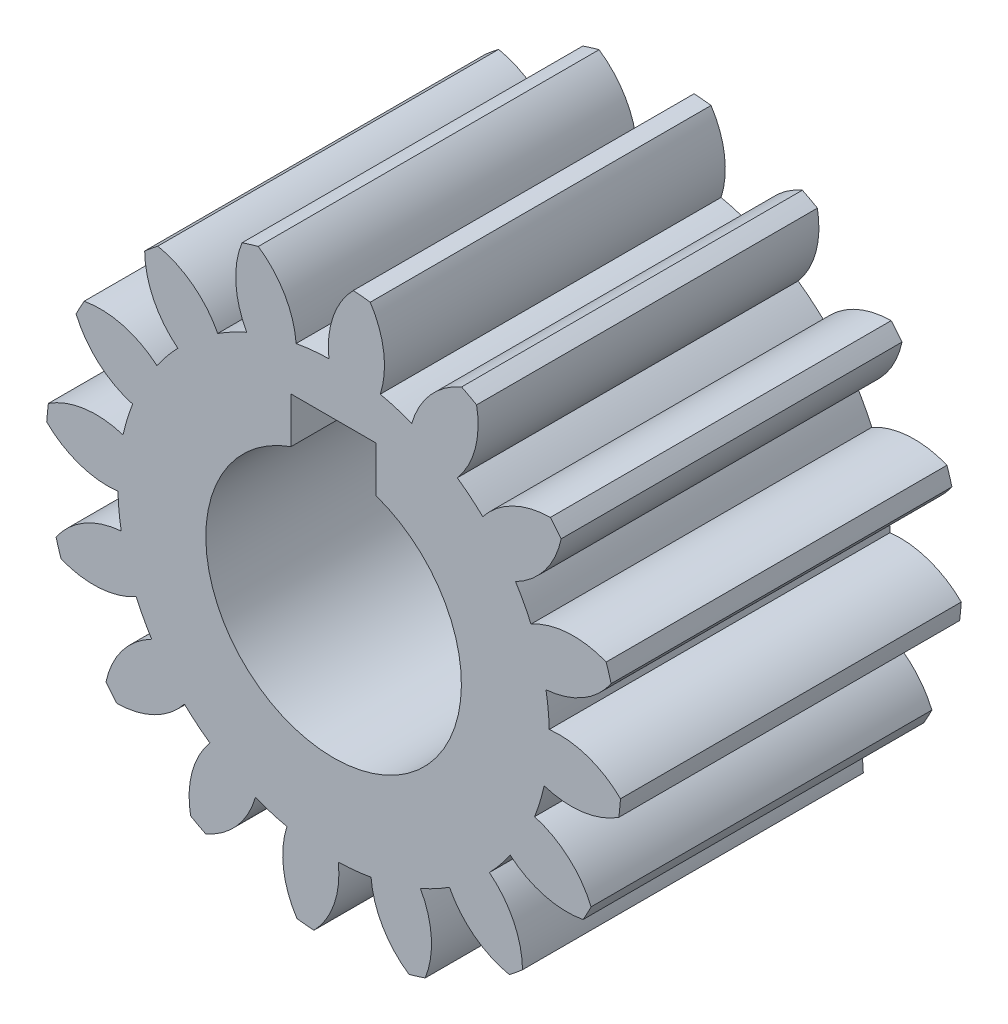
from build123d import *

# Parameters (mm, degrees)
SKETCH1_R           = 10.125
BOSS_EXTRUDE1_DEPTH = 16
BOSS_EXTRUDE2_START = -16
BOSS_EXTRUDE2_DEPTH = 16
CIRPATTERN1_COUNT   = 16
SKETCH3_R           = 6
SKETCH3_W           = 4
SKETCH3_H           = 3.6
CUT_EXTRUDE1_DEPTH  = 16


with BuildPart() as part:
    # Sketch1 → Boss-Extrude1 (new body)
    with BuildSketch(Plane.XY):
        Circle(SKETCH1_R)
    extrude(amount=BOSS_EXTRUDE1_DEPTH)

    # Sketch2 → Boss-Extrude2 (add)
    with BuildSketch(Plane.XY.offset(16).offset(BOSS_EXTRUDE2_START)):
        with BuildLine():
            ThreePointArc((2.190686363, 9.885166577), (2.352411056, 11.690772793), (1.720520144, 13.389914504))
            ThreePointArc((1.720520144, 13.389914504), (1.323231394, 13.43499381), (0.924781901, 13.468287881))
            ThreePointArc((0.924781901, 13.468287881), (-0.026453509, 11.925070502), (-0.220092608, 10.122607581))
            ThreePointArc((-0.220092608, 10.122607581), (0.992423546, 10.076245358), (2.190686363, 9.885166577))
        make_face()
    boss_extrude2 = extrude(amount=BOSS_EXTRUDE2_DEPTH)

    # CirPattern1: Boss-Extrude2 ×16 about axis
    cirpattern1_axis = Axis((0, 0, 0), (0, 0, 1))
    for i in range(1, CIRPATTERN1_COUNT):
        add(boss_extrude2.rotate(cirpattern1_axis, i * 360 / CIRPATTERN1_COUNT))

    # Sketch3 → Cut-Extrude1 (cut)
    with BuildSketch(Plane.XY.offset(16)):
        Circle(SKETCH3_R)
        with Locations((0, 6)):
            Rectangle(SKETCH3_W, SKETCH3_H)
    extrude(amount=-CUT_EXTRUDE1_DEPTH, mode=Mode.SUBTRACT)


solid = part.part
